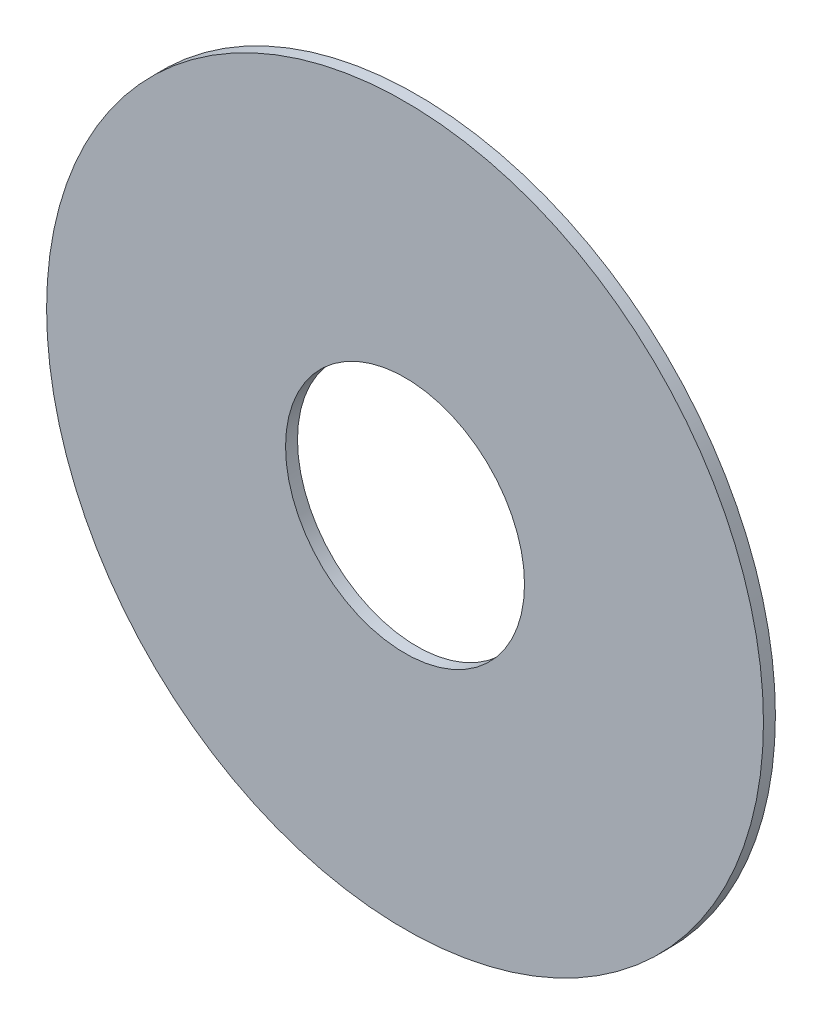
SolidWorks part; units mm, degrees
ref_plane "Front Plane" through (0, 0, 0) normal (0, 0, 1) x (1, 0, 0)
ref_plane "Top Plane" through (0, 0, 0) normal (0, 1, 0) x (1, 0, 0)
ref_plane "Right Plane" through (0, 0, 0) normal (1, 0, 0) x (0, 0, -1)
sketch "Sketch1" plane through (0, 0, 0) normal (0, 0, 1) x (1, 0, 0)
  circle A0 centre (0, 0) radius 30
  circle A1 centre (0, 0) radius 10
  dimension "D1" = 60
  dimension "D2" = 20
extrude "Boss-Extrude1" add sketch "Sketch1" along normal mid plane 1
